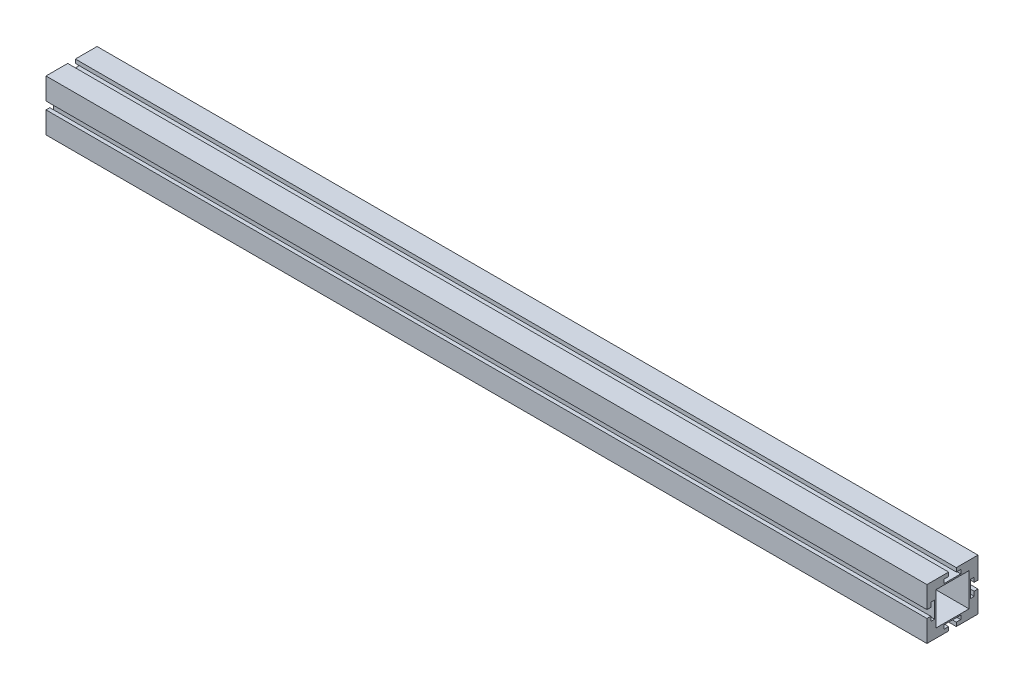
SolidWorks part; units mm, degrees
ref_plane "Front Plane" through (0, 0, 0) normal (0, 0, 1) x (1, 0, 0)
ref_plane "Top Plane" through (0, 0, 0) normal (0, 1, 0) x (1, 0, 0)
ref_plane "Right Plane" through (0, 0, 0) normal (1, 0, 0) x (0, 0, -1)
sketch "Sketch1" plane through (0, 0, 0) normal (1, 0, 0) x (0, 0, -1)
  line L0 (0, 0) -> (0, 33.8923) construction
  line L1 (-20, -20) -> (-3, -20)
  line L2 (-20, -20) -> (-20, -3)
  line L3 (-20, 20) -> (-3, 20)
  line L4 (20, -20) -> (20, -3)
  line L5 (-20, -20) -> (20, 20) construction
  line L6 (-20, 20) -> (20, -20) construction
  line L7 (-13, -13) -> (13, -13)
  line L8 (-13, -13) -> (-13, 13)
  line L9 (-13, 13) -> (13, 13)
  line L10 (13, -13) -> (13, 13)
  line L11 (-13, -13) -> (13, 13) construction
  line L12 (-13, 13) -> (13, -13) construction
  line L13 (0, 0) -> (25.505, 0) construction
  line L14 (17, 3) -> (17, 6.5)
  line L15 (-6.5, 17) -> (-3, 17)
  line L16 (6.5, 17) -> (6.5, 14)
  line L17 (3, 17) -> (6.5, 17)
  line L18 (-6.5, 14) -> (6.5, 14)
  line L19 (17, -6.5) -> (17, -3)
  line L20 (3, 20) -> (20, 20)
  line L21 (14, -6.5) -> (17, -6.5)
  line L22 (-3, 20) -> (-3, 17)
  line L23 (17, 3) -> (20, 3)
  line L24 (3, 20) -> (3, 17)
  line L25 (17, -3) -> (20, -3)
  line L26 (-20, 20) -> (20, 20) construction
  line L27 (14, -6.5) -> (14, 6.5)
  line L28 (-17, -17) -> (17, -17) construction
  line L29 (20, 3) -> (20, 20)
  line L30 (-6.5, 17) -> (-6.5, 14)
  line L31 (14, 6.5) -> (17, 6.5)
  line L32 (14, -14) -> (14, 14) construction
  line L33 (-14, 14) -> (14, 14) construction
  line L34 (-17, 17) -> (17, 17) construction
  line L35 (3, -20) -> (3, -17)
  line L36 (-17, -17) -> (-17, 17) construction
  line L37 (-14, -14) -> (-14, 14) construction
  line L38 (-14, -14) -> (14, -14) construction
  line L39 (17, -17) -> (17, 17) construction
  line L40 (20, -20) -> (20, 20) construction
  line L41 (3, -17) -> (6.5, -17)
  line L42 (6.5, -17) -> (6.5, -14)
  line L43 (-6.5, -14) -> (6.5, -14)
  line L44 (-6.5, -17) -> (-6.5, -14)
  line L45 (-6.5, -17) -> (-3, -17)
  line L46 (-3, -20) -> (-3, -17)
  line L47 (-14, -6.5) -> (-14, 6.5)
  line L48 (-14, -6.5) -> (-17, -6.5)
  line L49 (-17, -6.5) -> (-17, -3)
  line L50 (-17, -3) -> (-20, -3)
  line L51 (-17, 3) -> (-20, 3)
  line L52 (-17, 3) -> (-17, 6.5)
  line L53 (-14, 6.5) -> (-17, 6.5)
  line L54 (-20, 3) -> (-20, 20)
  line L55 (3, -20) -> (20, -20)
  line L56 (-20, -20) -> (-20, 20) construction
  line L58 (-20, -20) -> (20, -20) construction
  point P0 (0, 0)
  point P6 (0, 0)
  dimension "D1" = 40
  dimension "D2" = 40
  dimension "D3" = 26
  dimension "D4" = 26
  dimension "D7" = 3
  dimension "D8" = 3
  dimension "D9" = 6
  dimension "D10" = 13
  dimension "D11" = 3
  dimension "D12" = 6
  dimension "D13" = 13
  dimension "D5" = 3
  dimension "D6" = 3
extrude "Boss-Extrude1" add sketch "Sketch1" along normal blind 690
